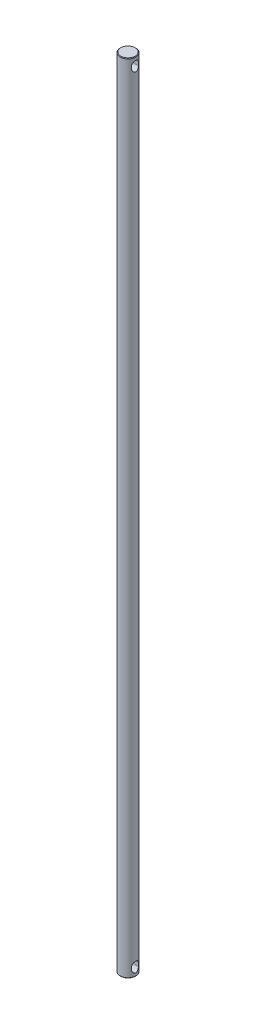
SolidWorks part; units mm, degrees
material "45#"
ref_plane "前基準面" through (0, 0, 0) normal (0, 0, 1) x (1, 0, 0)
ref_plane "上基準面" through (0, 0, 0) normal (0, 1, 0) x (1, 0, 0)
ref_plane "右基準面" through (0, 0, 0) normal (1, 0, 0) x (0, 0, -1)
sketch "草图1" plane through (0, 0, 0) normal (0, 1, 0) x (1, 0, 0)
  circle A0 centre (0, 0) radius 7
  dimension "D1" = 14
extrude "凸台-拉伸1" add sketch "草图1" along normal mid plane 715
chamfer "倒角1" distance 0.5 angle 45 2 edges at (0, -357.5, 7) (0, 357.5, 7)
sketch "草图2" plane through (0, 0, 0) normal (1, 0, 0) x (0, 0, -1)
  line L0 (0, -351.5) -> (0, -348.5) construction
  line L1 (-3, -351.5) -> (-3, -348.5)
  line L2 (3, -351.5) -> (3, -348.5)
  line L3 (-64.7029, 0) -> (0, 0) construction
  line L4 (-6.5, -357.5) -> (6.5, -357.5) construction
  line L5 (0, 351.5) -> (0, 348.5) construction
  line L6 (-3, 351.5) -> (-3, 348.5)
  line L7 (3, 351.5) -> (3, 348.5)
  arc A0 (-3, -351.5) -> (3, -351.5) centre (0, -351.5) ccw
  arc A1 (3, -348.5) -> (-3, -348.5) centre (0, -348.5) ccw
  arc A2 (-3, 351.5) -> (3, 351.5) centre (0, 351.5) cw
  arc A3 (3, 348.5) -> (-3, 348.5) centre (0, 348.5) cw
  point P3 (0, -350)
  point P15 (0, 350)
  dimension "D1" = 6
  dimension "D2" = 7.5
  dimension "D3" = 3
extrude "切除-拉伸1" cut sketch "草图2" against normal through all both and the other way through all
